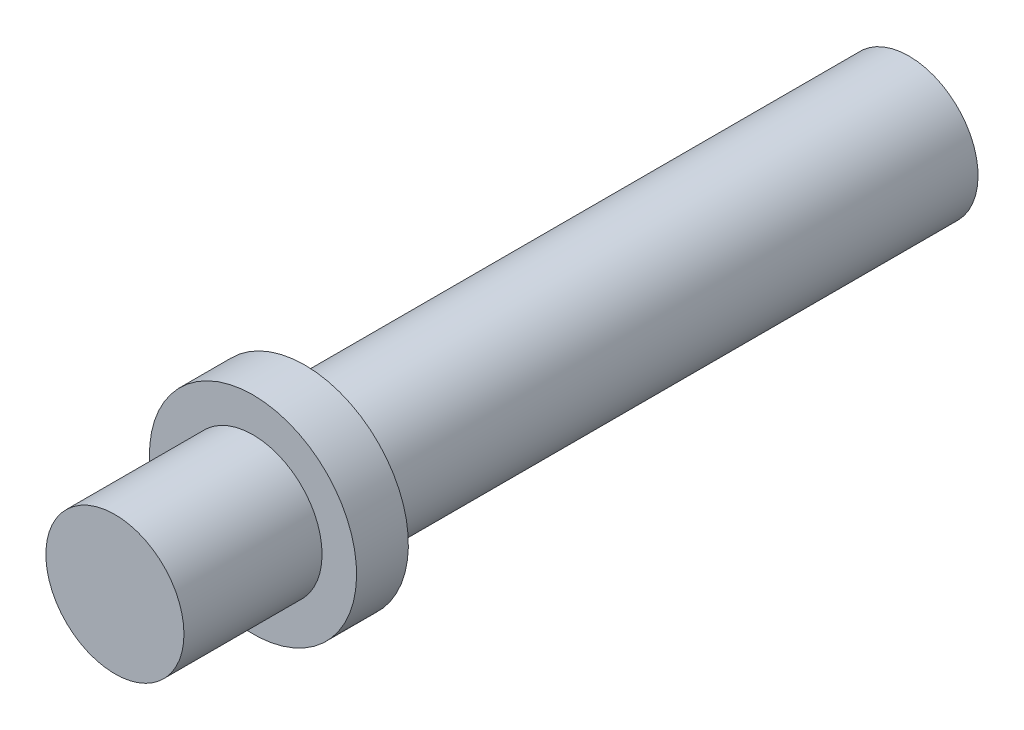
from build123d import *

# Parameters (mm, degrees)
SKETCH_1_R      = 4
EXTRUDE_1_DEPTH = 8
SKETCH_2_R      = 6
EXTRUDE_2_DEPTH = 3
SKETCH_3_R      = 4
EXTRUDE_3_DEPTH = 30
SKETCH_4_R      = 4
EXTRUDE_4_DEPTH = 5


with BuildPart() as part:
    # 草图1 → 凸台-拉伸1 (new body)
    with BuildSketch(Plane.XY):
        with Locations((-145.504664302, 180.568940096)):
            Circle(SKETCH_1_R)
    extrude(amount=-EXTRUDE_1_DEPTH)

    # 草图2 → 凸台-拉伸2 (add)
    with BuildSketch(Plane(origin=(0, 0, -8), x_dir=(-1, 0, 0), z_dir=(0, 0, -1))):
        with Locations(Location((145.504664302, 180.568940096, 0), (0, 0, 90))):
            Circle(SKETCH_2_R)
    extrude(amount=EXTRUDE_2_DEPTH)

    # 草图3 → 凸台-拉伸3 (add)
    with BuildSketch(Plane(origin=(0, 0, -11), x_dir=(-1, 0, 0), z_dir=(0, 0, -1))):
        with Locations(Location((145.504664302, 180.568940096, 0), (0, 0, 180))):
            Circle(SKETCH_3_R)
    extrude(amount=EXTRUDE_3_DEPTH)

    # 草图4 → 凸台-拉伸4 (add)
    with BuildSketch(Plane(origin=(0, 0, -41), x_dir=(-1, 0, 0), z_dir=(0, 0, -1))):
        with Locations(Location((145.504664302, 180.568940096, 0), (0, 0, 180))):
            Circle(SKETCH_4_R)
    extrude(amount=EXTRUDE_4_DEPTH)


solid = part.part
